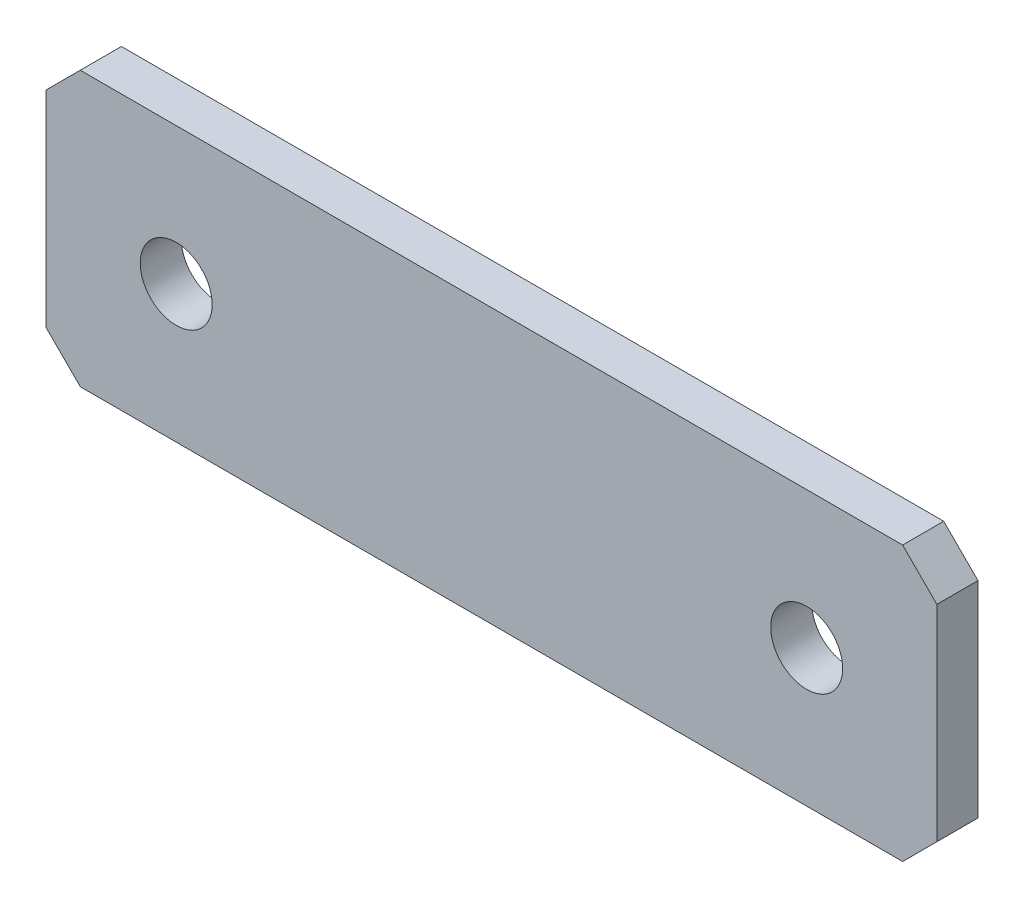
from build123d import *

# Parameters (mm, degrees)
SKETCH1_R           = 5.25
BOSS_EXTRUDE1_DEPTH = 3


with BuildPart() as part:
    # Sketch1 → Boss-Extrude1 (new, symmetric)
    with BuildSketch(Plane.XY):
        Polygon((-65, 15), (-60, 20), (60, 20), (65, 15), (65, -15), (60, -20), (-60, -20), (-65, -15), align=None)
        with Locations((-46, 0)):
            Circle(SKETCH1_R, mode=Mode.SUBTRACT)
        with Locations((46, 0)):
            Circle(SKETCH1_R, mode=Mode.SUBTRACT)
    extrude(amount=BOSS_EXTRUDE1_DEPTH, both=True)


solid = part.part
